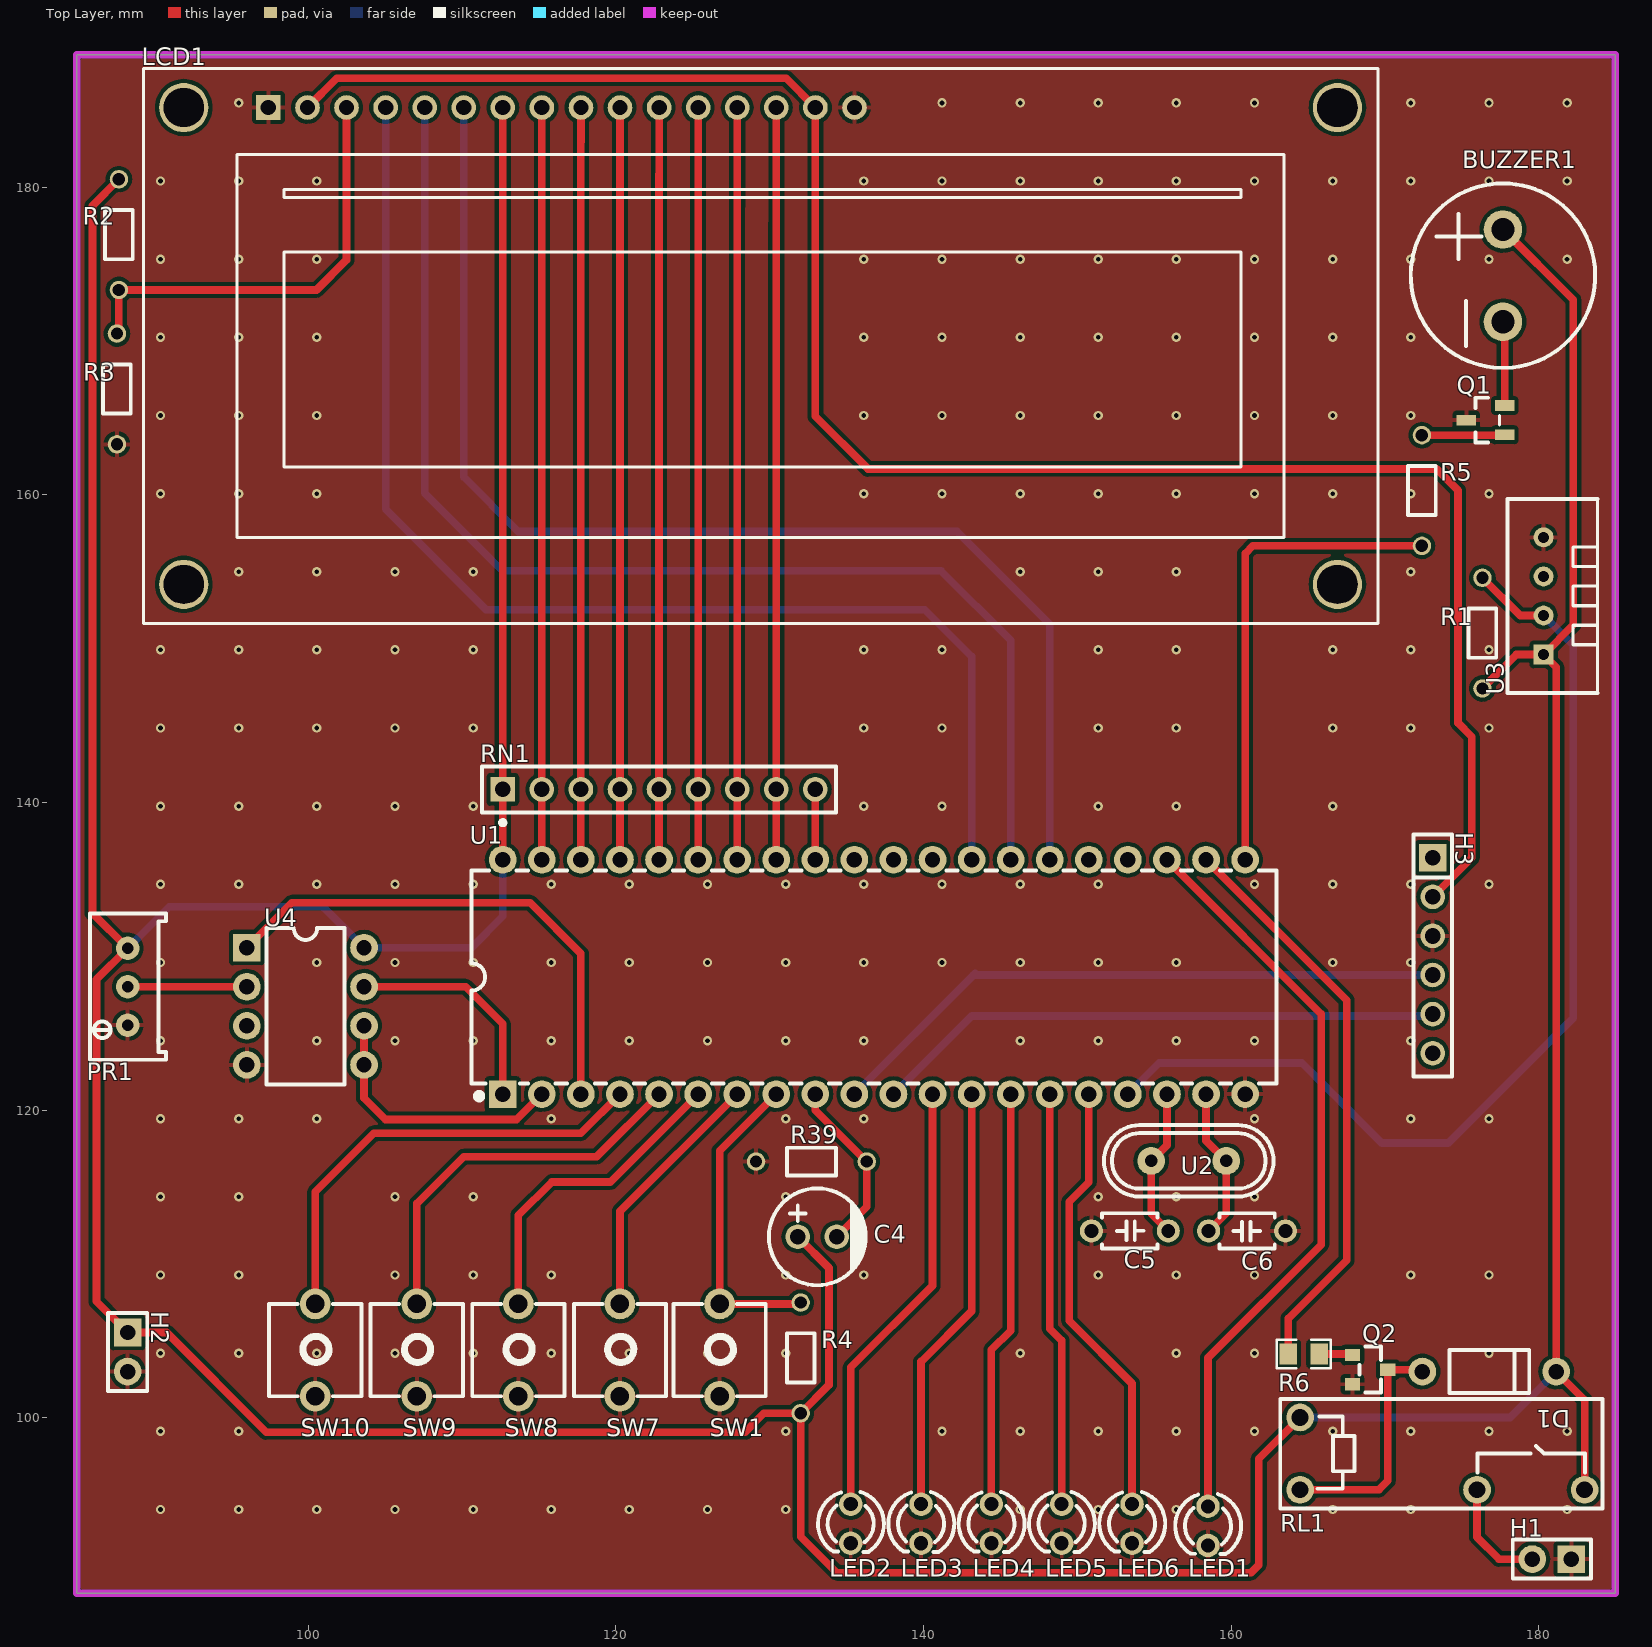
[diagram p0: Top Layer view]
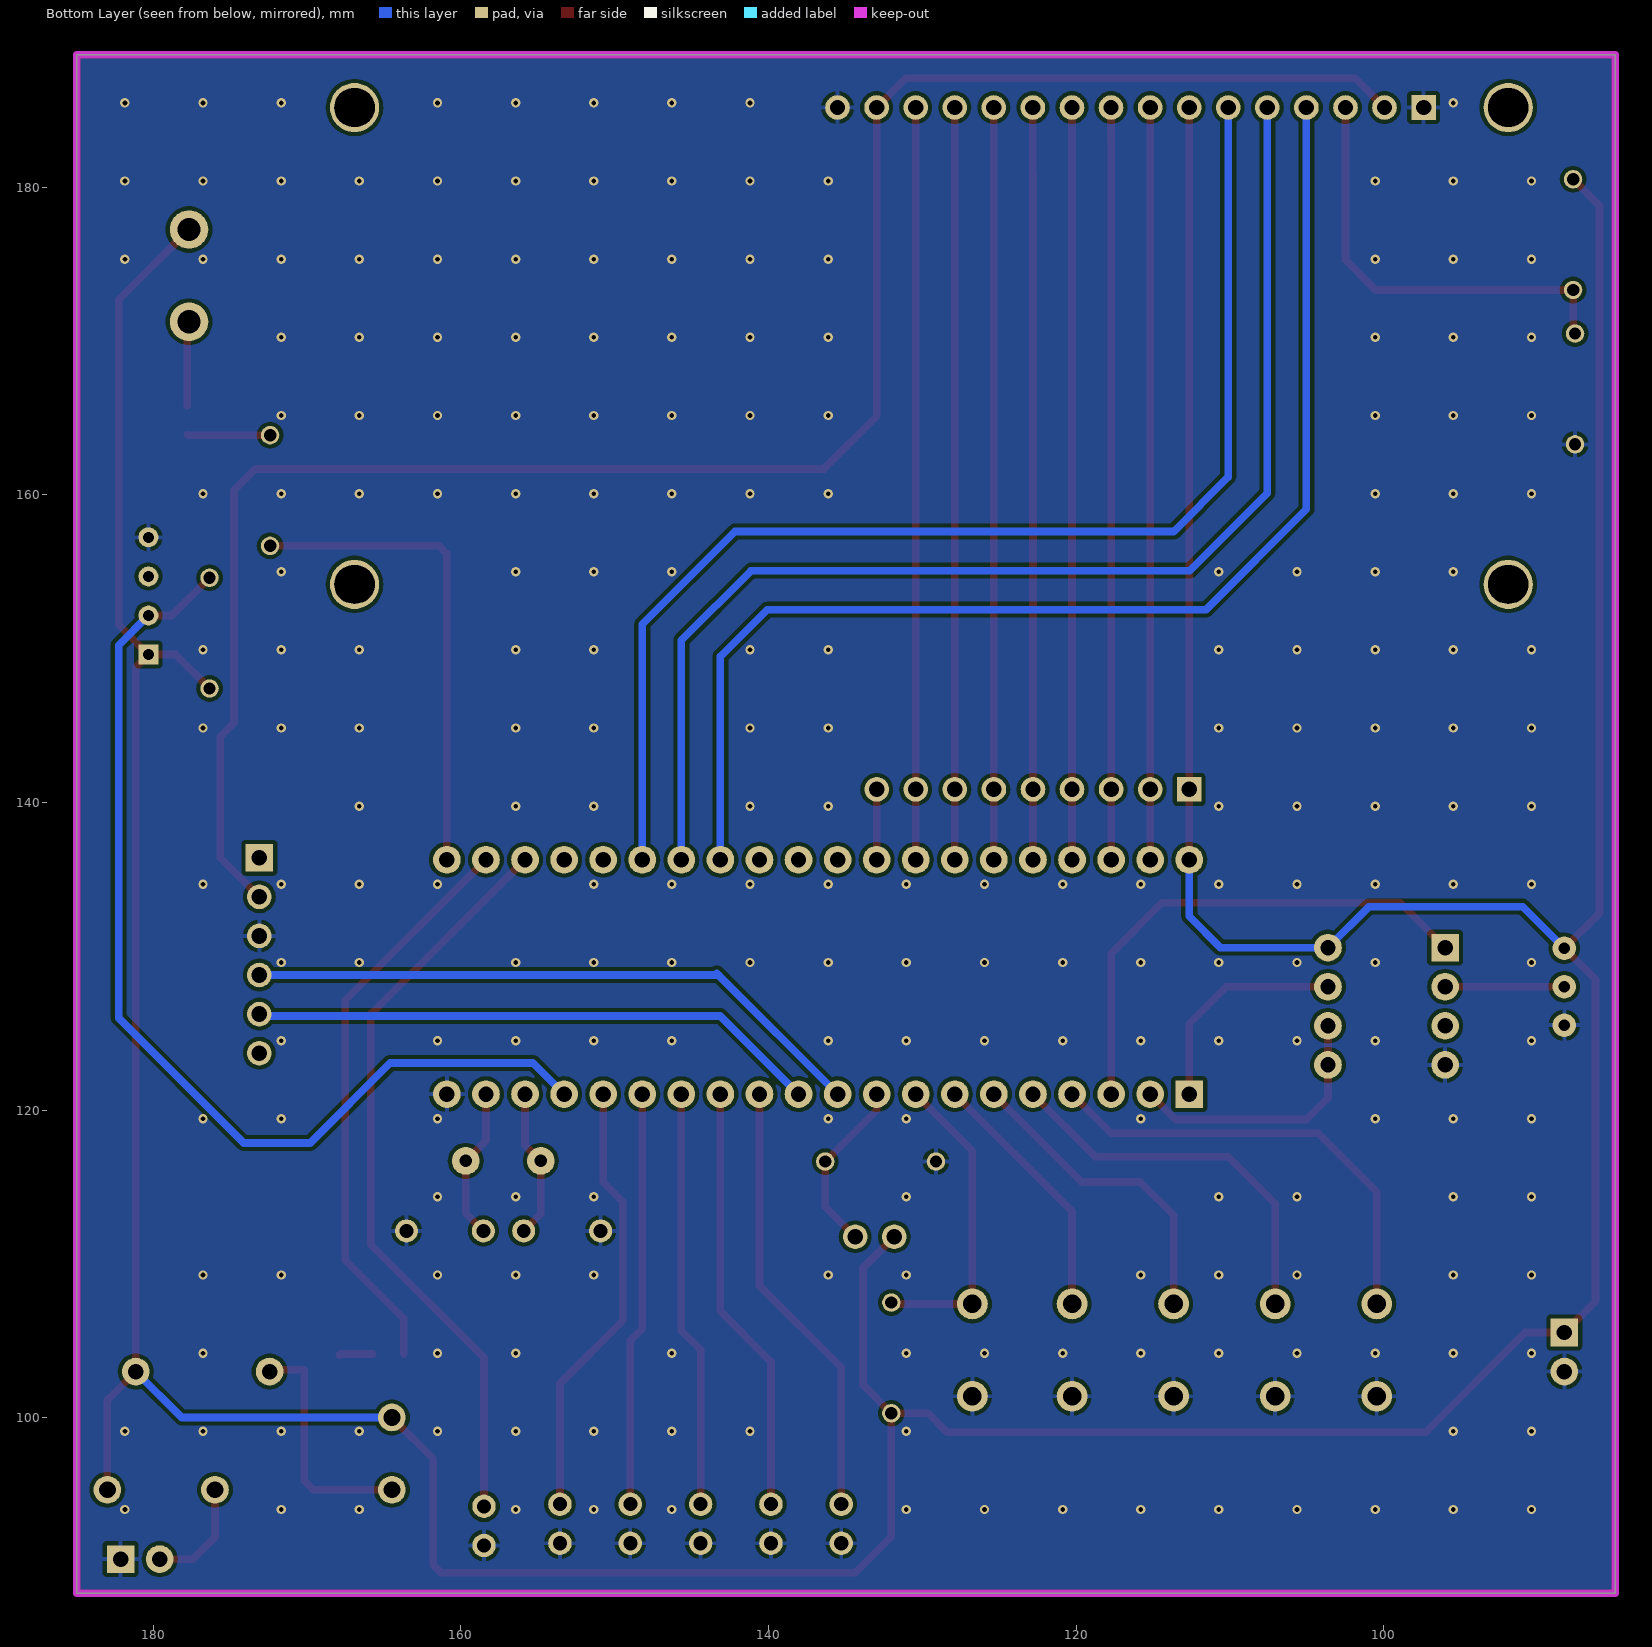
[diagram p1: Bottom Layer view, seen from below]
# Altium PCB MISC89128.pcbdoc
Units mm, origin at the board's own origin, x right, y up, seen from the top; angles counter-clockwise.
Board outline 100 x 100 mm, 2 copper layers (Top Layer, Bottom Layer), stack 1.58 mm thick; 36 components, 43 nets, 152 pads, 226 vias.

## Layer stack, top to bottom
Top Solder Mask Layer: solder mask 0.01, Dk 3.3
Top Layer: signal copper 0.035
Dielectric1: surface 1.51, FR4, Dk 4.5
Bottom Layer: signal copper 0.035
Bottom Solder Mask Layer: solder mask 0.01, Dk 3.3

## Board outline
84.963,188.595 84.963,88.595 184.963,88.595 184.963,188.595

## Design rules (kind name [scope] priority, off if disabled: settings)
BoardOutlineClearance copperThickness2oz_1 [All] p2 off: genericclearance=0.203 ignorepadtopadclearanceinfootprint=FALSE except(0: Arc-SplitContinuation Track-SplitContinuation SMDPad-SplitContinuation THPad-SplitContinuation Via-SplitContinuation Fill-SplitContinuation Region-SplitContinuation Poly-SplitContinuation Text-SplitContinuation Hole-SplitContinuation; 0.152: Arc-CutoutEdge Track-CutoutEdge SMDPad-CutoutEdge THPad-CutoutEdge Via-CutoutEdge Text-CutoutEdge; 0.175: Hole-OutlineEdge Hole-CutoutEdge; 0.254: Poly-OutlineEdge Poly-CutoutEdge; 0.3: Arc-OutlineEdge Track-OutlineEdge SMDPad-OutlineEdge THPad-OutlineEdge Via-OutlineEdge Fill-OutlineEdge Region-OutlineEdge Text-OutlineEdge Fill-CutoutEdge Region-CutoutEdge)
BoardOutlineClearance Plane_innerPlane_1 [All] p4 off: genericclearance=0.102 ignorepadtopadclearanceinfootprint=FALSE except(0: Arc-SplitContinuation Track-SplitContinuation SMDPad-SplitContinuation THPad-SplitContinuation Via-SplitContinuation Fill-SplitContinuation Region-SplitContinuation Poly-SplitContinuation Text-SplitContinuation Hole-SplitContinuation; 0.152: Arc-CutoutEdge Track-CutoutEdge SMDPad-CutoutEdge THPad-CutoutEdge Via-CutoutEdge Text-CutoutEdge; 0.175: Hole-OutlineEdge Hole-CutoutEdge; 0.254: Poly-OutlineEdge Poly-CutoutEdge; 0.3: Arc-OutlineEdge Track-OutlineEdge SMDPad-OutlineEdge THPad-OutlineEdge Via-OutlineEdge Fill-OutlineEdge Region-OutlineEdge Text-OutlineEdge Fill-CutoutEdge Region-CutoutEdge)
BoardOutlineClearance Copper_copperRegion_1 [All] p6 off: genericclearance=0.102 ignorepadtopadclearanceinfootprint=FALSE except(0: Arc-SplitContinuation Track-SplitContinuation SMDPad-SplitContinuation THPad-SplitContinuation Via-SplitContinuation Fill-SplitContinuation Region-SplitContinuation Poly-SplitContinuation Text-SplitContinuation Hole-SplitContinuation; 0.152: Arc-CutoutEdge Track-CutoutEdge SMDPad-CutoutEdge THPad-CutoutEdge Via-CutoutEdge Text-CutoutEdge; 0.175: Hole-OutlineEdge Hole-CutoutEdge; 0.254: Poly-OutlineEdge Poly-CutoutEdge; 0.3: Arc-OutlineEdge Track-OutlineEdge SMDPad-OutlineEdge THPad-OutlineEdge Via-OutlineEdge Fill-OutlineEdge Region-OutlineEdge Text-OutlineEdge Fill-CutoutEdge Region-CutoutEdge)
BoardOutlineClearance copperThickness1oz_1 [All] p8: genericclearance=0.102 ignorepadtopadclearanceinfootprint=FALSE except(0: Arc-SplitContinuation Track-SplitContinuation SMDPad-SplitContinuation THPad-SplitContinuation Via-SplitContinuation Fill-SplitContinuation Region-SplitContinuation Poly-SplitContinuation Text-SplitContinuation Hole-SplitContinuation; 0.152: Arc-CutoutEdge Track-CutoutEdge SMDPad-CutoutEdge THPad-CutoutEdge Via-CutoutEdge Text-CutoutEdge; 0.175: Hole-OutlineEdge Hole-CutoutEdge; 0.254: Poly-OutlineEdge Poly-CutoutEdge; 0.3: Arc-OutlineEdge Track-OutlineEdge SMDPad-OutlineEdge THPad-OutlineEdge Via-OutlineEdge Fill-OutlineEdge Region-OutlineEdge Text-OutlineEdge Fill-CutoutEdge Region-CutoutEdge)
Clearance copperThickness2oz [All] p1 off: gap=0.203 ignorepadtopadclearanceinfootprint=FALSE except(0.152: SMDPad-Track SMDPad-SMDPad THPad-Track SMDPad-THPad THPad-THPad Track-Via SMDPad-Via THPad-Via Via-Via Fill-SMDPad Region-SMDPad Fill-THPad Region-THPad Fill-Via Region-Via Fill-Fill Fill-Region Region-Region Arc-Track Arc-SMDPad Arc-THPad Arc-Via Fill-Arc Region-Arc Arc-Arc Text-Track SMDPad-Text Text-THPad Text-Via Fill-Text Region-Text Arc-Text Text-Text; 0.175: Hole-Track Hole-SMDPad Hole-THPad Hole-Via Fill-Hole Region-Hole Hole-Arc Hole-Text; 0.254: Poly-Track Poly-SMDPad Poly-THPad Poly-Via Poly-Fill Poly-Region Poly-Poly Poly-Arc Poly-Text Poly-Hole; 0.3: Fill-Track Region-Track)
Clearance Plane_innerPlane [All] p3 off: gap=0.102 ignorepadtopadclearanceinfootprint=FALSE except(0.152: SMDPad-Track SMDPad-SMDPad THPad-Track SMDPad-THPad THPad-THPad Track-Via SMDPad-Via THPad-Via Via-Via Fill-SMDPad Region-SMDPad Fill-THPad Region-THPad Fill-Via Region-Via Fill-Fill Fill-Region Region-Region Arc-Track Arc-SMDPad Arc-THPad Arc-Via Fill-Arc Region-Arc Arc-Arc Text-Track SMDPad-Text Text-THPad Text-Via Fill-Text Region-Text Arc-Text Text-Text; 0.175: Hole-Track Hole-SMDPad Hole-THPad Hole-Via Fill-Hole Region-Hole Hole-Arc Hole-Text; 0.254: Poly-Track Poly-SMDPad Poly-THPad Poly-Via Poly-Fill Poly-Region Poly-Poly Poly-Arc Poly-Text Poly-Hole; 0.3: Fill-Track Region-Track)
Clearance Copper_copperRegion [All] p5 off: gap=0.102 ignorepadtopadclearanceinfootprint=FALSE except(0.152: SMDPad-Track SMDPad-SMDPad THPad-Track SMDPad-THPad THPad-THPad Track-Via SMDPad-Via THPad-Via Via-Via Fill-SMDPad Region-SMDPad Fill-THPad Region-THPad Fill-Via Region-Via Fill-Fill Fill-Region Region-Region Arc-Track Arc-SMDPad Arc-THPad Arc-Via Fill-Arc Region-Arc Arc-Arc Text-Track SMDPad-Text Text-THPad Text-Via Fill-Text Region-Text Arc-Text Text-Text; 0.175: Hole-Track Hole-SMDPad Hole-THPad Hole-Via Fill-Hole Region-Hole Hole-Arc Hole-Text; 0.254: Poly-Track Poly-SMDPad Poly-THPad Poly-Via Poly-Fill Poly-Region Poly-Poly Poly-Arc Poly-Text Poly-Hole; 0.3: Fill-Track Region-Track)
Clearance copperThickness1oz [All] p7: gap=0.102 ignorepadtopadclearanceinfootprint=FALSE except(0.152: SMDPad-Track SMDPad-SMDPad THPad-Track SMDPad-THPad THPad-THPad Track-Via SMDPad-Via THPad-Via Via-Via Fill-SMDPad Region-SMDPad Fill-THPad Region-THPad Fill-Via Region-Via Fill-Fill Fill-Region Region-Region Arc-Track Arc-SMDPad Arc-THPad Arc-Via Fill-Arc Region-Arc Arc-Arc Text-Track SMDPad-Text Text-THPad Text-Via Fill-Text Region-Text Arc-Text Text-Text; 0.175: Hole-Track Hole-SMDPad Hole-THPad Hole-Via Fill-Hole Region-Hole Hole-Arc Hole-Text; 0.254: Poly-Track Poly-SMDPad Poly-THPad Poly-Via Poly-Fill Poly-Region Poly-Poly Poly-Arc Poly-Text Poly-Hole; 0.3: Fill-Track Region-Track)
DiffPairsRouting differentialPair [All] p1: maxlimit=0.152 minlimit=0.152 mostfreqgap=0.152 toplayer_minwidth=0.127 toplayer_prefwidth=0.254 toplayer_maxwidth=2.54 toplayer_mingap=0.152 toplayer_prefgap=0.152 toplayer_maxgap=0.152 bottomlayer_minwidth=0.127 bottomlayer_prefwidth=0.254 bottomlayer_maxwidth=2.54 bottomlayer_mingap=0.152 bottomlayer_prefgap=0.152 bottomlayer_maxgap=0.152 maxuncoupledlength=0.254
HoleToHoleClearance otherClearance [All] p1: gap=0.3 allowstackedmicrovias=TRUE
Length netLength [All] p1: minlimit=0 maxlimit=0
PasteMaskExpansion pasteMaskExpansion [All] p1: expansion=0
PlaneConnect innerPlane [All] p1: planeconnectstyle=Relief reliefexpansion=0.508 reliefentries=4 reliefconductorwidth=0.254 reliefairgap=0.254
PolygonConnect copperRegion [All] p1: connectstyle=Relief reliefconductorwidth=0.254 reliefentries=4 polygonreliefangle="90 Angle" airgapwidth=0.254 via.connectstyle=Relief via.reliefconductorwidth=0.254 via.reliefentries=4 via.polygonreliefangle="90 Angle" via.airgapwidth=0.254
RoutingVias viaSize [All] p1: holewidth=0.305 width=0.61 viastyle="Through Hole" minholewidth=0.3 minwidth=0.5 maxholewidth=6.3 maxwidth=10
SolderMaskExpansion solderMaskExpansion [IsVia] p1: expansion=-25.4 istentingtop=TRUE
SolderMaskExpansion solderMaskExpansion [All] p2: expansion=0.051 istentingtop=FALSE
Width copperThickness2oz_2 [All] p1 off: maxlimit=2.54 minlimit=0.203 preferedwidth=0.254
Width copperThickness1oz_2 [All] p2: maxlimit=2.54 minlimit=0.127 preferedwidth=0.254

## Components (designator, comment, footprint, x,y, rotation, side; value= is the part's Value field where it differs from the comment)
BUZZER1 "buzzer" BUZ-TH_BD12.0-P6.00-D0.9-RD 177.673,174.244 r90 top
C4 "10uF" CAP-TH_BD6.3-P2.50-D1.0-FD 133.096,111.76 r0 top
C5 "30pF" CAP-TH_L3.6-W2.3-P5.00-D0.5 153.416,112.141 r0 top
C6 "30pF" CAP-TH_L3.6-W2.3-P5.00-D0.5 161.036,112.141 r180 top
D1 "" DO_1N4007 176.784,102.997 r180 top
H1 "" HDR-TH_2P-P2.54-V-M-1 180.848,90.805 r180 top
H2 "" HDR-TH_2P-P2.54-V-M-1 88.265,104.267 r270 top
H3 "" HDR-TH_6P-P2.54-V-F 173.101,130.048 r270 top
LCD1 "HS1602A" LCD1602 129.413,169.672 r0 top
LED1 "" LED_TH-3mm 158.496,92.964 r270 top
LED2 "" LED_TH-3mm 135.27,93.106 r270 top
LED3 "" LED_TH-3mm 139.842,93.106 r270 top
LED4 "" LED_TH-3mm 144.414,93.106 r270 top
LED5 "" LED_TH-3mm 148.986,93.106 r270 top
LED6 "" LED_TH-3mm 153.558,93.106 r270 top
PR1 "10kΩ" R_3296 88.138,128.016 r90 top
Q1 "" S8550P_SOT 176.498,164.847 r0 top
Q2 "" S8050_SOT-23 169.037,103.124 r180 top
R1 "10kΩ" Res_1/8W 176.276,151.003 r270 top
R2 "10kΩ" Res_1/8W 87.757,176.911 r90 top
R3 "1kΩ" Res_1/8W 87.63,166.878 r90 top
R4 "10kΩ" Res_1/8W 131.953,103.886 r270 top
R5 "2.2kΩ" Res_1/8W 172.339,160.274 r270 top
R6 "1K" R0805 164.719,104.14 r180 top
R39 "10kΩ" Res_1/8W 132.715,116.586 r0 top
RL1 "HT46F-DC12V-SHAG" RELAY-TH_HT46F-DCXXV-SHAG 173.736,97.663 r0 top
RN1 "-" RES-ARRAY-TH_9P-P2.54-D1.0 122.809,140.843 r0 top
SW1 "Tact switch, 6*6*5 plastic head, 260G, travel 0.25mm, through-hole 2-pin" KEY-TH_2P-L6.0-W6.0-P5.00 126.746,104.394 r90 top
SW7 "Tact switch, 6*6*5 plastic head, 260G, travel 0.25mm, through-hole 2-pin" KEY-TH_2P-L6.0-W6.0-P5.00 120.269,104.394 r90 top
SW8 "Tact switch, 6*6*5 plastic head, 260G, travel 0.25mm, through-hole 2-pin" KEY-TH_2P-L6.0-W6.0-P5.00 113.665,104.394 r90 top
SW9 "Tact switch, 6*6*5 plastic head, 260G, travel 0.25mm, through-hole 2-pin" KEY-TH_2P-L6.0-W6.0-P5.00 107.061,104.394 r90 top
SW10 "Tact switch, 6*6*5 plastic head, 260G, travel 0.25mm, through-hole 2-pin" KEY-TH_2P-L6.0-W6.0-P5.00 100.457,104.394 r90 top
U1 "STC89C52" DIP-40_L52.3-W13.9-P2.54-LS15.2-BL 136.779,128.651 r0 top
U2 "12MHz" HC-49US_L11.0-W4.6-P4.88 157.244,116.695 r0 top
U3 "DHT11" SENSOR-TH_DHT11 180.314,153.42 r90 top
U4 "ADC0832CCN" DIP-8_L9.7-W6.4-P2.54-LS7.6-BL 99.822,126.746 r270 top

## Footprints (in the part's own frame and the unit in brackets; to place one, negate y for a bottom-side part, rotate by r counter-clockwise, add the part's x,y. Pads: shape width x height; smd on the part's side, far side on the other; paste and mask are expansions set on the pad)
BUZ-TH_BD12.0-P6.00-D0.9-RD [mm]
  round 2.5 hole 1.5 paste+0 mask+0.05: 1(-3,0) 2(3,0)
  silkscreen extent -5.99,-5.99 5.99,5.99
CAP-TH_BD6.3-P2.50-D1.0-FD [mm]
  round 1.6 hole 1: 1(-1.27,0) 2(1.27,0)
  silkscreen extent -3.15,-3.15 3.17,3.15
CAP-TH_L3.6-W2.3-P5.00-D0.5 [mm]
  round 1.5 hole 0.9: 1(-2.5,0) 2(2.5,0)
  silkscreen extent -1.8,-1.15 1.8,1.15
DIP-8_L9.7-W6.4-P2.54-LS7.6-BL [mm]
  rect 1.8x1.8 hole 1 paste+0 mask+0.05: 1(-3.81,-3.81)
  round 1.8 hole 1 paste+0 mask+0.05: 2(-1.27,-3.81) 3(1.27,-3.81) 4(3.81,-3.81) 5(3.81,3.81) 6(1.27,3.81) 7(-1.27,3.81) 8(-3.81,3.81)
  silkscreen extent -5.08,-2.53 5.08,2.53
DIP-40_L52.3-W13.9-P2.54-LS15.2-BL [mm]
  rect 1.8x1.8 hole 1: 1(-24.13,-7.62)
  round 1.8 hole 1: 2(-21.59,-7.62) 3(-19.05,-7.62) 4(-16.51,-7.62) 5(-13.97,-7.62) 6(-11.43,-7.62) 7(-8.89,-7.62) 8(-6.35,-7.62) 9(-3.81,-7.62) 10(-1.27,-7.62) 11(1.27,-7.62) 12(3.81,-7.62) 13(6.35,-7.62) 14(8.89,-7.62) 15(11.43,-7.62) 16(13.97,-7.62) 17(16.51,-7.62) 18(19.05,-7.62) 19(21.59,-7.62) 20(24.13,-7.62) 21(24.13,7.62) 22(21.59,7.62) 23(19.05,7.62) 24(16.51,7.62) 25(13.97,7.62) 26(11.43,7.62) 27(8.89,7.62) 28(6.35,7.62) 29(3.81,7.62) 30(1.27,7.62) 31(-1.27,7.62) 32(-3.81,7.62) 33(-6.35,7.62) 34(-8.89,7.62) 35(-11.43,7.62) 36(-13.97,7.62) 37(-16.51,7.62) 38(-19.05,7.62) 39(-21.59,7.62) 40(-24.13,7.62)
  silkscreen extent -26.16,-7.95 26.16,6.93
DO_1N4007 [mm]
  round 1.8 hole 1 paste+0 mask+0.051: 1(-4.35,0) 2(4.35,0)
  silkscreen extent -2.6,-1.4 2.6,1.4
HC-49US_L11.0-W4.6-P4.88 [mm]
  round 1.8 hole 0.8: 1(-2.44,0) 2(2.44,0)
  silkscreen extent -5.51,-2.32 5.51,2.32
HDR-TH_2P-P2.54-V-M-1 [mm]
  rect 1.8x1.8 hole 1: 1(-1.27,0)
  round 1.8 hole 1: 2(1.27,0)
  silkscreen extent -2.54,-1.27 2.54,1.27
HDR-TH_6P-P2.54-V-F [mm]
  rect 1.8x1.8 hole 1.02: 1(-6.35,0)
  round 1.6 hole 1.02: 2(-3.81,0) 3(-1.27,0) 4(1.27,0) 5(3.81,0) 6(6.35,0)
  silkscreen extent -7.87,-1.25 7.87,1.25
KEY-TH_2P-L6.0-W6.0-P5.00 [mm]
  round 2 hole 1.2: 1(-3,0) 2(3,0)
  silkscreen extent -3,-3 3,3
LCD1602 [mm]
  round 3.2 hole 2.5 slot 2.625 at 0 deg: 0(-37.5,-15.5) 0(-37.5,15.5) 0(37.5,-15.5) 0(37.5,15.5)
  rect 1.6x1.6 hole 1: 1(-32,15.5)
  round 1.6 hole 1: 2(-29.46,15.5) 3(-26.92,15.5) 4(-24.38,15.5) 5(-21.84,15.5) 6(-19.3,15.5) 7(-16.76,15.5) 8(-14.22,15.5) 9(-11.68,15.5) 10(-9.14,15.5) 11(-6.6,15.5) 12(-4.06,15.5) 13(-1.52,15.5) 14(1.02,15.5) 15(3.56,15.5) 16(6.1,15.5)
  silkscreen extent -40.13,-18.03 40.13,18.03
LED_TH-3mm [mil]
  round 60 hole 36 paste+0 mask+2: 1(-50,0) 2(50,0)
  silkscreen extent -81,-84 72,85
R0805 [mm]
  rect 1.133x1.377 smd paste-100 mask+0.051: 1(-1,0) 2(1,0)
  silkscreen extent -1.76,-0.92 1.76,0.92
R_3296 [mil]
  round 60 hole 30 paste+0 mask+2: 1(-98.4,-5) 2(0,-5) 3(98.4,-5)
  silkscreen extent -187,-103 187,92
RELAY-TH_HT46F-DCXXV-SHAG [mm]
  round 1.8 hole 1.1: 1(-9.25,2.35) 2(-9.25,-2.35) 3(2.25,-2.35) 4(9.25,-2.35)
  silkscreen extent -10.54,-3.56 10.41,3.56
RES-ARRAY-TH_9P-P2.54-D1.0 [mm]
  rect 1.6x1.6 hole 1: 1(-10.16,0)
  round 1.6 hole 1: 2(-7.62,0) 3(-5.08,0) 4(-2.54,0) 5(0,0) 6(2.54,0) 7(5.08,0) 8(7.62,0) 9(10.16,0)
  silkscreen extent -11.5,-2.31 11.5,1.5
Res_1/8W [mil]
  round 47.2 hole 31.5 paste+0 mask+2: 1(-141.7,2.48) 2(141.7,2.48)
  silkscreen extent -63,-33 63,38
S8050_SOT-23 [mm]
  rect 1x0.8 smd paste+0 mask+0.051: 1(1.15,-0.95) 2(1.15,0.95) 3(-1.15,0)
  silkscreen extent -0.7,-1.5 0.7,1.5
S8550P_SOT [mm]
  rect 1.25x0.701 smd paste+0 mask+0.051: 1(1.291,-0.95) 2(1.291,0.95) 3(-1.208,0)
  silkscreen extent -0.61,-1.46 0.94,1.46
SENSOR-TH_DHT11 [mil]
  rect 51x51 hole 28: 1(-150,0)
  round 51 hole 28: 2(-50,0) 3(50,0) 4(150,0)
  silkscreen extent -248,-138 248,93

## Via types
v1: diameter 0.61, hole 0.305, Top Layer to Bottom Layer, 226 vias

## Nets (pads, with @x,y where several pads share a name; then routed paths per layer and width w, separated by ;. In a path a pad name is that pad's centre, name@x,y a point inside that pad or via, vN(x,y) a via of type N, cw(c..) or ccw(c..) an arc to the next point about the centre after c; other vN are vias at no path point)
31: LED1.1 U1.23 | length 49.2
  Top Layer w0.5: U1.23 165.862,126.238 165.862,111.252 158.496,103.886 LED1.1
32: LED2.1 U1.12 | length 28.9
  Top Layer w0.5: LED2.1 135.27,103.266 140.589,108.585 U1.12
33: LED3.1 U1.13 | length 28
  Top Layer w0.5: LED3.1 139.842,103.647 143.129,106.934 U1.13
34: LED4.1 U1.14 | length 27.2
  Top Layer w0.5: LED4.1 144.414,104.409 145.669,105.664 U1.14
35: LED5.1 U1.15 | length 27
  Top Layer w0.5: U1.15 148.209,105.791 148.986,105.014 LED5.1
36: LED6.1 U1.16 | length 28.9
  Top Layer w0.5: U1.16 150.749,115.316 149.479,114.046 149.479,106.299 153.558,102.22 LED6.1
37: R1.1 U1.17 U3.2 | length 67.3
  Top Layer w0.5: R1.1 178.791,152.15 U3.2
  Bottom Layer w0.5: U1.17 155.321,123.063 164.592,123.063 169.799,117.856 174.117,117.856 182.245,125.984 182.245,150.22 U3.2
$1N1586: RN1.9 U1.32 | length 4.6
  Top Layer w0.5: U1.32 RN1.9
$1N1590: LCD1.8 RN1.2 U1.39 | length 48.9
  Top Layer w0.5: U1.39 RN1.2 115.189,183.987 115.193,183.991 LCD1.8
$1N1591: LCD1.9 RN1.3 U1.38 | length 48.9
  Top Layer w0.5: U1.38 RN1.3 117.729,182.935 117.733,182.939 LCD1.9
$1N1592: LCD1.10 RN1.4 U1.37 | length 48.9
  Top Layer w0.5: U1.37 RN1.4 120.269,181.883 120.273,181.887 LCD1.10
$1N1593: LCD1.11 RN1.5 U1.36 | length 48.9
  Top Layer w0.5: U1.36 RN1.5 122.809,180.831 122.813,180.835 LCD1.11
$1N1594: LCD1.12 RN1.6 U1.35 | length 48.9
  Top Layer w0.5: U1.35 RN1.6 125.349,179.779 125.353,179.783 LCD1.12
$1N1595: LCD1.13 RN1.7 U1.34 | length 48.9
  Top Layer w0.5: U1.34 RN1.7 127.889,178.727 127.893,178.731 LCD1.13
$1N1596: LCD1.14 RN1.8 U1.33 | length 48.9
  Top Layer w0.5: U1.33 RN1.8 130.429,177.674 130.433,177.678 LCD1.14
$1N1611: C5.2 U1.18 U2.1 | length 9.8
  Top Layer w0.5: U1.18 155.829,117.719 U2.1 154.804,113.253 C5.2
$1N1612: C6.2 U1.19 U2.2 | length 9.9
  Top Layer w0.5: U1.19 158.369,118.01 U2.2 159.684,113.289 C6.2
$1N1662: C4.2 R39.2 U1.9 | length 11.5
  Top Layer w0.5: U1.9 132.969,119.994 R39.2 136.314,113.708 C4.2
$1N14609: SW9.2 U1.5 | length 25.2
  Top Layer w0.5: SW9.2 107.061,113.919 110.109,116.967 118.745,116.967 U1.5
$1N14610: SW7.2 U1.7 | length 16.8
  Top Layer w0.5: SW7.2 120.269,113.411 U1.7
$1N14611: SW8.2 U1.6 | length 20.7
  Top Layer w0.5: SW8.2 113.665,113.157 115.824,115.316 119.634,115.316 U1.6
$1N14649: LCD1.3 R2.1 R3.2 | length 28.4
  Top Layer w0.5: R3.2 87.694,170.604 R2.1 100.541,173.312 102.493,175.264 LCD1.3
$1N14662: PR1.2 U4.2 | length 7.7
  Top Layer w0.5: PR1.2 U4.2
$1N14670: BUZZER1.1 Q1.2 | length 5.5
  Top Layer w0.5: BUZZER1.1 177.789,171.128 Q1.2
$1N14672: R4.1 SW1.2 U1.8 | length 20.5
  Top Layer w0.5: U1.8 126.746,117.348 SW1.2 131.925,107.394 R4.1
$1N14676: Q1.1 R5.1 | length 5.4
  Top Layer w0.5: R5.1 177.765,163.873 Q1.1
$1N14677: R5.2 U1.21 | length 31.6
  Top Layer w0.5: U1.21 160.909,156.175 161.409,156.675 R5.2
$1N14678: H3.4 U1.10 | length 40.9
  Bottom Layer w0.5: U1.10 143.256,128.778 ; 143.359,128.881 143.256,128.778 ; H3.4 143.256,128.778
$1N14679: H3.5 U1.11 | length 37.1
  Bottom Layer w0.5: U1.11 143.129,126.111 H3.5@173.078,126.111
$1N14681: R6.2 U1.22 | length 37.5
  Top Layer w0.5: U1.22 167.513,127.127 167.513,110.236 163.719,106.442 R6.2
$1N14683: Q2.1 R6.1 | length 2.2
  Top Layer w0.5: R6.1 167.821,104.14 Q2.1
$1N14685: D1.2 Q2.3 RL1.2 | length 15.5
  Top Layer w0.5: RL1.2 169.608,95.313 170.187,95.892 Q2.3 172.307,103.124 D1.2
$1N14691: H1.2 RL1.3 | length 7.3
  Top Layer w0.5: RL1.3 175.986,92.238 177.419,90.805 H1.2
$1N14693: SW10.2 U1.4 | length 29.7
  Top Layer w0.5: SW10.2 100.457,114.681 104.267,118.491 117.729,118.491 U1.4
+5V: BUZZER1.2 C4.1 D1.1 H2.1 LCD1.7 PR1.3 R1.2 R2.2 R4.2 RL1.1 RL1.4 RN1.1 U1.40 U3.1 U4.8 | length 376.6
  Top Layer w0.5: R2.2 85.979,178.795 85.979,132.801 PR1.3 86.233,128.483 86.233,107.569 H2.1 90.805,105.537 97.282,99.06 128.397,99.06 129.624,100.287 R4.2 ; U1.40 RN1.1 112.649,185.168 LCD1.7 ; C4.1 133.858,109.728 133.858,102.129 R4.2 ; RL1.1 161.798,97.325 161.798,90.424 161.29,89.916 134.366,89.916 132.016,92.266 R4.2 ; R1.2 178.545,149.61 U3.1 ; BUZZER1.2 182.245,172.672 182.245,151.541 U3.1 ; RL1.4 182.986,101.145 D1.1 181.134,148.791 U3.1
  Bottom Layer w0.5: PR1.3 90.973,133.223 100.965,133.223 U4.8 110.617,130.556 112.649,132.588 U1.40 ; RL1.1 178.15,100.013 D1.1
EN: LCD1.6 U1.26 | length 81.4
  Bottom Layer w0.5: LCD1.6 110.113,161.159 113.665,157.607 142.185,157.607 148.209,151.583 U1.26
GND: C5.1 C6.1 H1.1 H2.2 H3.3 LCD1.1 LCD1.16 LED1.2 LED2.2 LED3.2 LED4.2 LED5.2 LED6.2 PR1.1 Q1.3 Q2.2 R3.1 R39.1 SW1.1 SW7.1 SW8.1 SW9.1 SW10.1 U1.20 U3.4 U4.4
  other v1: 90.401,94.033 95.481,94.033 100.561,94.033 105.641,94.033 110.721,94.033 115.801,94.033 120.881,94.033 125.961,94.033 131.041,94.033 146.281,94.033 151.361,94.033 156.441,94.033 166.601,94.033 171.681,94.033 181.841,94.033 90.401,99.113 95.481,99.113 131.041,99.113 141.201,99.113 146.281,99.113 151.361,99.113 156.441,99.113 161.521,99.113 166.601,99.113 171.681,99.113 176.761,99.113 181.841,99.113 90.401,104.193 95.481,104.193 100.561,104.193 105.641,104.193 110.721,104.193 115.801,104.193 120.881,104.193 125.961,104.193 131.041,104.193 146.281,104.193 156.441,104.193 161.521,104.193 176.761,104.193 90.401,109.273 95.481,109.273 105.641,109.273 110.721,109.273 115.801,109.273 131.041,109.273 136.121,109.273 151.361,109.273 156.441,109.273 161.521,109.273 171.681,109.273 176.761,109.273 90.401,114.353 95.481,114.353 105.641,114.353 110.721,114.353 131.041,114.353 151.361,114.353 156.441,114.353 161.521,114.353 90.401,119.433 95.481,119.433 100.561,119.433 115.801,119.433 131.041,119.433 136.121,119.433 161.521,119.433 171.681,119.433 176.761,119.433 90.401,124.513 100.561,124.513 105.641,124.513 110.721,124.513 115.801,124.513 120.881,124.513 125.961,124.513 131.041,124.513 136.121,124.513 146.281,124.513 151.361,124.513 156.441,124.513 161.521,124.513 171.681,124.513 90.401,129.593 100.561,129.593 105.641,129.593 110.721,129.593 115.801,129.593 120.881,129.593 125.961,129.593 131.041,129.593 136.121,129.593 141.201,129.593 146.281,129.593 151.361,129.593 156.441,129.593 166.601,129.593 171.681,129.593 90.401,134.673 95.481,134.673 100.561,134.673 105.641,134.673 110.721,134.673 115.801,134.673 120.881,134.673 125.961,134.673 131.041,134.673 136.121,134.673 141.201,134.673 146.281,134.673 151.361,134.673 161.521,134.673 166.601,134.673 171.681,134.673 176.761,134.673 90.401,139.753 95.481,139.753 100.561,139.753 105.641,139.753 110.721,139.753 136.121,139.753 141.201,139.753 151.361,139.753 156.441,139.753 166.601,139.753 90.401,144.833 95.481,144.833 100.561,144.833 105.641,144.833 110.721,144.833 136.121,144.833 141.201,144.833 151.361,144.833 156.441,144.833 166.601,144.833 171.681,144.833 176.761,144.833 90.401,149.913 95.481,149.913 100.561,149.913 105.641,149.913 110.721,149.913 136.121,149.913 141.201,149.913 151.361,149.913 156.441,149.913 166.601,149.913 171.681,149.913 176.761,149.913 95.481,154.993 100.561,154.993 105.641,154.993 110.721,154.993 146.281,154.993 151.361,154.993 156.441,154.993 171.681,154.993 90.401,160.073 95.481,160.073 100.561,160.073 136.121,160.073 141.201,160.073 146.281,160.073 151.361,160.073 156.441,160.073 161.521,160.073 166.601,160.073 171.681,160.073 176.761,160.073 90.401,165.153 95.481,165.153 100.561,165.153 136.121,165.153 141.201,165.153 146.281,165.153 151.361,165.153 156.441,165.153 161.521,165.153 166.601,165.153 171.681,165.153 90.401,170.233 95.481,170.233 100.561,170.233 136.121,170.233 141.201,170.233 146.281,170.233 151.361,170.233 156.441,170.233 161.521,170.233 166.601,170.233 171.681,170.233 90.401,175.313 95.481,175.313 100.561,175.313 136.121,175.313 141.201,175.313 146.281,175.313 151.361,175.313 156.441,175.313 161.521,175.313 166.601,175.313 171.681,175.313 176.761,175.313 181.841,175.313 90.401,180.393 95.481,180.393 100.561,180.393 136.121,180.393 141.201,180.393 146.281,180.393 151.361,180.393 156.441,180.393 161.521,180.393 166.601,180.393 171.681,180.393 176.761,180.393 181.841,180.393 95.481,185.473 141.201,185.473 146.281,185.473 151.361,185.473 156.441,185.473 161.521,185.473 171.681,185.473 176.761,185.473 181.841,185.473
P10: U1.1 U4.7 | length 14.6
  Top Layer w0.5: U4.7 110.236,128.016 112.649,125.603 U1.1
P11: U1.2 U4.5 U4.6 | length 17.5
  Top Layer w0.5: U4.6 U4.5 103.632,120.777 105.029,119.38 113.538,119.38 U1.2
P12: U1.3 U4.1 | length 33.4
  Top Layer w0.5: U4.1 98.933,133.477 114.427,133.477 117.729,130.175 U1.3
RS: LCD1.4 U1.28 | length 81.4
  Bottom Layer w0.5: LCD1.4 105.033,159.055 111.561,152.527 140.081,152.527 143.129,149.479 U1.28
RW: LCD1.5 U1.27 | length 81.4
  Bottom Layer w0.5: LCD1.5 107.573,160.107 112.613,155.067 141.133,155.067 145.669,150.531 U1.27
VCC: H3.2 LCD1.2 LCD1.15 | length 126.3
  Top Layer w0.5: LCD1.2 101.852,187.071 131.074,187.071 LCD1.15 132.973,165.096 136.398,161.671 173.355,161.671 174.752,160.274 174.752,145.161 175.641,144.272 175.641,136.398 H3.2
pads on no net: H3.1 H3.6 LCD1.0 U1.24 U1.25 U1.29 U1.30 U1.31 U3.3 U4.3

## Polygon pours and split planes (outlines as drawn)
GND on Bottom Layer (solid, remove dead copper, pour order 2): 76.2,196.469 76.2,76.2 198.12,76.2 198.12,196.469
GND on Top Layer (solid, remove dead copper, pour order 0): 79.121,193.04 79.121,82.677 191.643,82.677 191.643,193.04

## Keep-outs
Board Outline Layer:
  the board outline again, w0.5